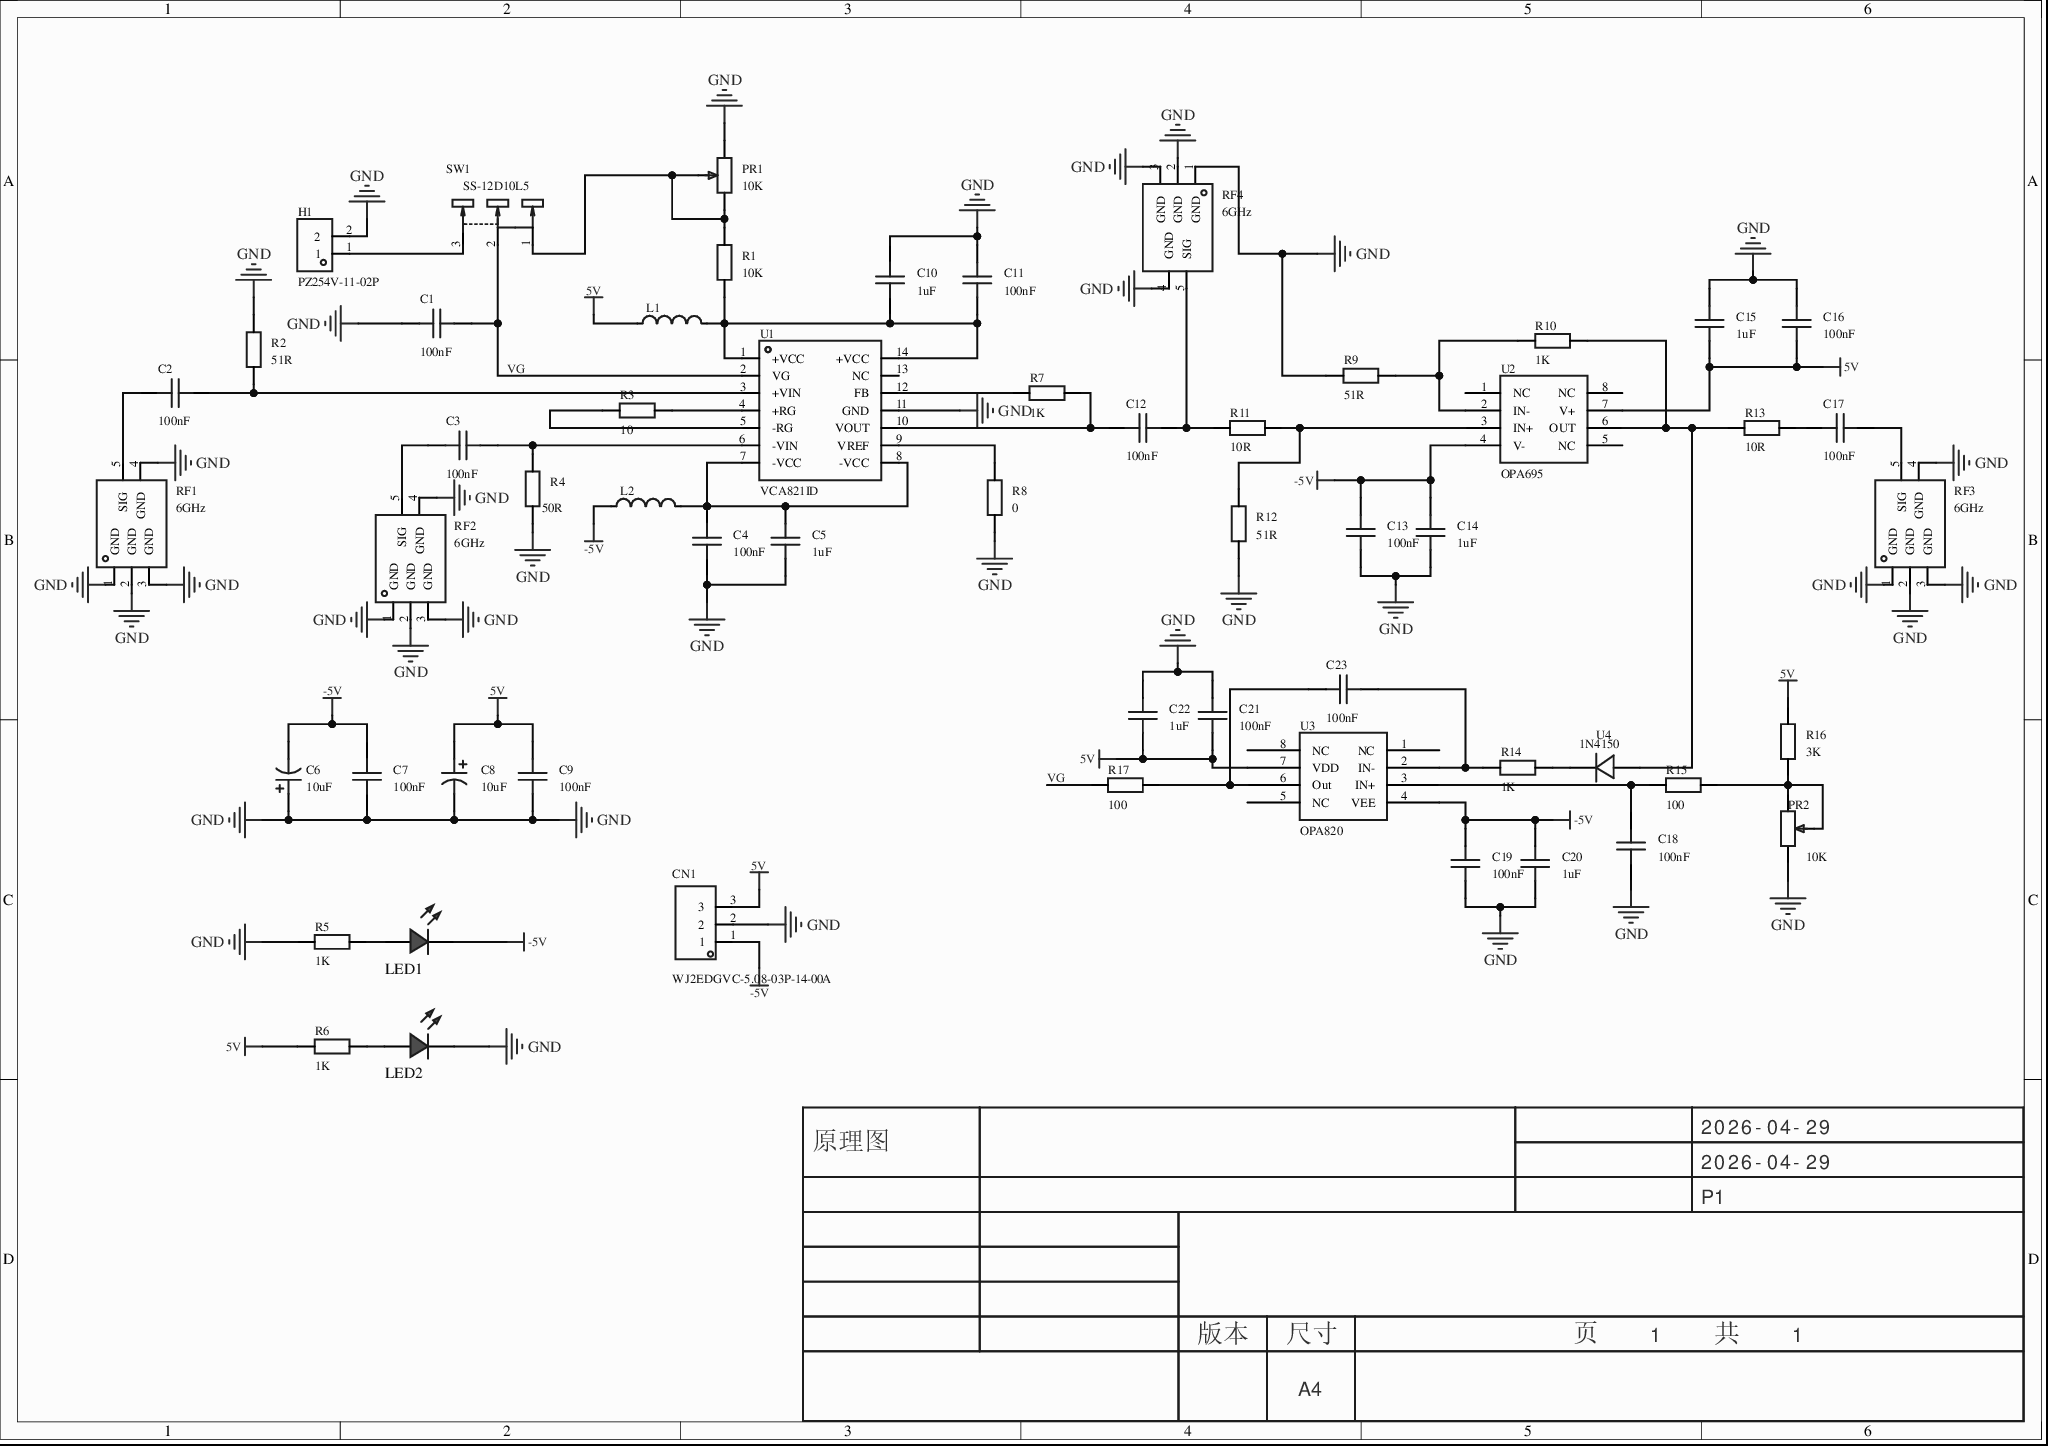
[diagram p0: MISC52012-3.schdoc]
# Altium project MISC52012-2.PrjPcb
1 sheet, 57 parts. Net scope: global (net labels, ports and power ports of the same name join across sheets).
Board file: MISC52012.pcbdoc

## Sheet MISC52012-3.schdoc
size 297 x 209 mm; Version: V1.0; @Project Name: MISC52012; @Page Count: 1; @Update Date: 2026-04-29; @Create Date: 2026-04-29; @Schematic Name: MISC52012; @Page No: 1; @Board Name: MISC52012; @Create Time: 22:58:53; @Update Time: 22:58:53; Size: A4

### Parts
C1  100nF  [C0603]
C2  100nF  [C0603]
C3  100nF  [C0603]
C4  100nF  [C0603]
C5  1uF  [C0603]
C6  10uF  [CAP-TH_BD5.0-P2.00-D0.5-FD-A]
C7  100nF  [C0603]
C8  10uF  [CAP-TH_BD5.0-P2.00-D0.5-FD-A]
C9  100nF  [C0603]
C10  1uF  [C0603]
C11  100nF  [C0603]
C12  100nF  [C0603]
C13  100nF  [C0603]
C14  1uF  [C0603]
C15  1uF  [C0603]
C16  100nF  [C0603]
C17  100nF  [C0603]
C18  100nF  [C0603]
C19  100nF  [C0603]
C20  1uF  [C0603]
C21  100nF  [C0603]
C22  1uF  [C0603]
C23  100nF  [C0603]
CN1  WJ2EDGVC-5.08-03P-14-00A  [CONN-TH_3P-P5.08-WJ2EDGVC-3P]
H1  PZ254V-11-02P  [HDR-TH_2P-P2.54-V-M]
L1  10uH  [L0603]  (value not drawn)
L2  10uH  [L0603]  (value not drawn)
LED1  (no value)  [LED_0603]
LED2  (no value)  [LED_0603]
PR1  10K  [R_3386P]
PR2  10K  [R_3386P]
R1  10K  [R0603]
R2  51R  [R0603]
R3  10  [R0603]
R4  50R  [R0603]
R5  1K  [R0603]
R6  1K  [R0603]
R7  1K  [R0603]
R8  0  [R0603]
R9  51R  [R0603]
R10  1K  [R0603]
R11  10R  [R0603]
R12  51R  [R0603]
R13  10R  [R0603]
R14  1K  [R0603]
R15  100  [R0603]
R16  3K  [R0603]
R17  100  [R0603]
RF1  6GHz  [SMA-SMD_BWSMA-KE-P001]
RF2  6GHz  [SMA-SMD_BWSMA-KE-P001]
RF3  6GHz  [SMA-SMD_BWSMA-KE-P001]
RF4  6GHz  [SMA-SMD_BWSMA-KE-P001]
SW1  SS-12D10L5  [SW-TH_SS-12D10L5]
U1  VCA821ID  [SOIC-14_L8.7-W3.9-P1.27-LS6.0-BL]
U2  OPA695  [SOIC-8]
U3  OPA820  [SOP8]
U4  1N4150  [SOD-123_L2.7-W1.6-LS3.7-RD-1]

### Nets
5V: C8.1 C9.2 C15.1 C16.1 C21.1 C22.1 CN1.3 L1.1 R6.1 R16.2 U2.7(V+) U3.7(VDD)
-5V: C6.2 C7.2 C13.2 C14.2 C19.2 C20.2 CN1.1 L2.1 LED1.1(C) U2.4(V-) U3.4(VEE)
GND: C1.1 C4.2 C5.1 C6.1 C7.1 C8.2 C9.1 C10.2 C11.2 C13.1 C14.1 C15.2 C16.2 C18.1 C19.1 C20.1 C21.2 C22.2 CN1.2 H1.2 LED2.1(C) PR1.1 PR2.1 R2.2 R4.1 R5.1 R8.1 R9.1 R12.1 RF1.1(GND) RF1.2(GND) RF1.3(GND) RF1.4(GND) RF2.1(GND) RF2.2(GND) RF2.3(GND) RF2.4(GND) RF3.1(GND) RF3.2(GND) RF3.3(GND) RF3.4(GND) RF4.1(GND) RF4.2(GND) RF4.3(GND) RF4.4(GND) U1.11(GND)
VG: C1.2 R17.1 SW1.2 U1.2(VG)
NetC2_1: C2.1 RF1.5(SIG)
NetC2_2: C2.2 R2.1 U1.3(+VIN)
NetC3_1: C3.1 RF2.5(SIG)
NetC3_2: C3.2 R4.2 U1.6(-VIN)
NetC4_1: C4.1 C5.2 L2.2 U1.7(-VCC) U1.8(-VCC)
NetC10_1: C10.1 C11.1 L1.2 R1.1 U1.1(+VCC) U1.14(+VCC)
NetC12_1: C12.1 R7.2 U1.10(VOUT)
NetC12_2: C12.2 R11.1 RF4.5(SIG)
NetC17_1: C17.1 R13.2
NetC17_2: C17.2 RF3.5(SIG)
NetC18_2: C18.2 R15.1 U3.3(IN+)
NetC23_1: C23.1 R14.1 U3.2(IN-)
NetC23_2: C23.2 R17.2 U3.6(Out)
NetH1_1: H1.1 SW1.3
NetLED1_2: LED1.2(A) R5.2
NetLED2_2: LED2.2(A) R6.2
NetPR1_2: PR1.2 PR1.3 R1.2 SW1.1
NetPR2_2: PR2.2 PR2.3 R15.2 R16.1
NetR3_1: R3.1 U1.5(-RG)
NetR3_2: R3.2 U1.4(+RG)
NetR7_1: R7.1 U1.12(FB)
NetR8_2: R8.2 U1.9(VREF)
NetR9_2: R9.2 R10.1 U2.2(IN-)
NetR10_2: R10.2 R13.1 U2.6(OUT) U4.2(A)
NetR11_2: R11.2 R12.2 U2.3(IN+)
NetR14_2: R14.2 U4.1(K)

Not connected (* = marked no-connect by the designer): U1 13(NC)*; U2 1(NC)* 5(NC)* 8(NC)*; U3 1(NC)* 5(NC)* 8(NC)*

### Notes on the sheet
- 2026-04-29
- 原理图
- P1
- 版本
- 尺寸
- A4
- 页    1    共    1

### Library data of the parts
C1-C5 C7 C9-C16 = CAP_0603: ConvertToPcb: yes; SymbolName: Capacitance; ModelId: ac125912035d415993ca9572d50418b1; ModelName: C0603_L1.6-W0.8-H0.8; ModelTransform: 62.992,31.496,0,0,0,0,0,0,0; Device: CAP_0603; AddInBom: yes; Supplier Footprint: 0603; FootprintName: C0603
  C1-C4 C7 C9 C11-C13 C16: Value: 100nF
  C5 C10 C14 C15: Value: 1uF
C6 C8 = ERG50V10M5X11: 容值:10uF;精度:±20%;额定电压:50V;纹波电流:180mA@100kHz;等效串联电阻(ESR):1.3Ω@100kHz;; Manufacturer: JIERR(捷而瑞); AddInBom: yes; ModelId: 230b3bd6484f4b52b9cf74c8bd6c6199; ModelTransform: 197.2437,197.23953,0,0,0,0,0,0,-196.85; Tolerance: ±20%; Voltage Rating: 50V; Pin Spacing: 2mm; Lifetime: 2000hrs@105℃; Symbol: ERG50V10M5X11; Device: ERG50V10M5X11; LCSC Part Name: 10uF ±20% 50V; SupplierPart: C47344184; ManufacturerPart: ERG50V10M5X11; Supplier Footprint: 插件,D5xL11mm; Datasheet: https://item.szlcsc.com/datasheet/ERG50V10M5X11/49556625.html; Supplier: LCSC; ConvertToPcb: yes; FootprintName: CAP-TH_BD5.0-P2.00-D0.5-FD-A; ModelName: CAP-TH_BD5.0-P2.00-D0.5-FD-A; Value: 10uF; Ripple Current: 180mA@100kHz; Equivalent Series Resistance(ESR): 1.3Ω@100kHz; Diameter: 5mm; Height - Seated (Max): 11mm; Operating Temperature: -40℃~+105℃
C17-C23 = CL10B104KB8NNNC: 容值:100nF;精度:±10%;额定电压:50V;温度系数:X7R;; Manufacturer: SAMSUNG(三星); AddInBom: yes; ModelId: ac125912035d415993ca9572d50418b1; ModelName: C0603_L1.6-W0.8-H0.8; ModelTransform: 62.992,31.496,0,0,0,0,0,0,0; Tolerance: ±10%; Voltage Rating: 50V; Temperature Coefficient: X7R; Symbol: CL10B104KB8NNNC; Device: CL10B104KB8NNNC; LCSC Part Name: 100nF ±10% 50V; ManufacturerPart: CL10B104KB8NNNC; Supplier Footprint: 0603; JLCPCB Part Class: Extended Part; Datasheet: https://item.szlcsc.com/datasheet/CL10B104KB8NNNC/1943.html; Supplier: LCSC; ConvertToPcb: yes; FootprintName: C0603
  C17-C19 C21 C23: SupplierPart: C1591; Value: 100nF
  C20 C22: Value: 1uF
CN1 = WJ2EDGVC-5.08-03P-14-00A: 连接器类型:板端/插座-闭口;固定方式:卡扣固定;结构:1x3P;间距:5.08mm;颜色:绿色;安装方式:直插;排数:1;每排PIN数:3;额定电流:10A;额定电压:300V;线规 - AWG:-;线规 - 平方毫米:-;工作温度:-40℃~+105℃;; Manufacturer: KANGNEX(康奈克斯电气); Symbol: WJ2EDGVC-3P; AddInBom: yes; ModelId: e882f8e8ed7147e981563fc403497786; ModelTransform: 674.8018,326.771,0,0,0,0,0,17.323,-157.48; Number of Positions or Pins: 1x3P; Pitch: 5.08mm; Number of PINs Per Row: 3; Current Rating: 10A; Voltage Rating (Max): 300V; Device: WJ2EDGVC-5.08-03P-14-00A; LCSC Part Name: 卡扣固定 1x3P 5.08mm 排数:1 每排P数:3; SupplierPart: C8412; ManufacturerPart: WJ2EDGVC-5.08-03P-14-00A; Supplier Footprint: 插件,P=5.08mm; JLCPCB Part Class: 扩展库; Datasheet: https://item.szlcsc.com/datasheet/WJ2EDGVC-5.08-03P-14-00A/8906.html; Supplier: LCSC; ConvertToPcb: yes; FootprintName: CONN-TH_3P-P5.08-WJ2EDGVC-3P; ModelName: CONN-TH_3P-P5.08-WJ2EDGVC-3P; Connector Type: 板端/插座-闭口; Termination Style: 卡扣固定; Color: 绿色; Mounting Type: 直插; Number of Pins: 3P; Number of Rows: 1; Wire Gauge - AWG: -; Wire Gauge - mm2: -; Operating Temperature: -40℃~+105℃; Connection Type: -; Outlet Direction (Vertical Basis): -
H1 = PZ254V-11-02P: 插针结构:1x2P;间距:2.54mm;行距:-;圆针/方针:方针;安装方式:直插;排数:单排;总PIN位数:2P;额定电流:3A;额定电压:250V;配合针长度:6mm;塑高:2.5mm;端接针长度:3mm;触头材质:黄铜;触头镀层:-;工作温度:-40℃~+105℃;颜色:黑色;; Manufacturer: XFCN(兴飞); AddInBom: yes; ModelId: e35305ec3aa84b66b849f914b715e73f; ModelName: HDR2.54-M-LI-1X2P; ModelTransform: 200,100,0,0,0,0,0,0,-118.11; Pin Structure: 1x2P; Pitch: 2.54mm; Circluar Pins/Square Pins: 方针; Current Rating: 3A; Voltage Rating (Max): 250V; Symbol: PZ254V-11-02P; Device: PZ254V-11-02P; LCSC Part Name: 1x2P 间距:2.54mm 方针 直插; SupplierPart: C492401; ManufacturerPart: PZ254V-11-02P; Supplier Footprint: 插件,P=2.54mm; Datasheet: https://item.szlcsc.com/datasheet/PZ254V-11-02P/502957.html; Supplier: LCSC; ConvertToPcb: yes; FootprintName: HDR-TH_2P-P2.54-V-M; Row Spacing: -; Mounting Type: 直插; Number of Rows: 单排; Number of Pins: 2P; Length of Mating Pin: 6mm; Insulation Height: 2.5mm; Length of End Connection Pin: 3mm; Contact Material: 黄铜; Contact Plating: -; Operating Temperature: -40℃~+105℃; Color: 黑色
L1 L2 = L_0603: Symbol: SDFL1608S100KTF; AddInBom: yes; ModelId: 2bc5ec593d464d6ba9807aec0b5673c2; ModelName: L0603_L1.6-W0.8-H0.5_BEAD; ModelTransform: 62.992,31.496,0,180,0,0,0.094,0.629,0; Device: L_0603; Supplier Footprint: L0603; ConvertToPcb: yes; FootprintName: L0603; Value: 10uH
LED1 LED2 = LED_0603-R: Symbol: LED_R; Convert to PCB: yes; 3D Model: dd8257b0d61a4cd7b68939a056e08095; 3D Model Transform: 58.72,29.4,22.03,0,0,0,0,0,0; ModelName: LED-0603_R; Device: LED_0603-R; Add into BOM: yes; Supplier Footprint: 0603; FootprintName: LED_0603
PR1 PR2 = R_3386P: Symbol: 3386P-1-103LF; ConvertToPcb: yes; ModelId: 6a25d8a4450b4318959c1cd98efa6b0c0819f05c4eef4c71ace90d822a990e87; ModelName: RES-ADJ-TH_3P-L9.5-W9.5-P2.54-BR-BS; ModelTransform: 375.19,375.19,387,-90,0,0,0,0,-197; Device: R_3386P; AddInBom: yes; FootprintName: R_3386P; Value: 10K; Supplier Footprint: 直插
R1-R17 = Res_0603: ConvertToPcb: yes; SymbolName: 电阻; ModelId: fc143cca1e79419f9cd78b61e9279f08; ModelTransform: 31.8897,63.7794,0,90,0,0,0,0,0; Device: Res_0603; AddInBom: yes; Supplier Footprint: 0603; FootprintName: R0603; ModelName: R0603
  R1: Value: 10K
  R2 R9 R12: Value: 51R
  R3: Value: 10
  R4: Value: 50R
  R5-R7 R10 R14: Value: 1K
  R8: Value: 0
  R11 R13: Value: 10R
  R15 R17: Value: 100
  R16: Value: 3K
RF1-RF4 = SMA-KHD9A: 连接器类型:板端;接口类型:内孔;端口数量:1;接口长度/高度:8mm;频率:6GHz;射频系列:SMA;阻抗:50Ω;样式:偏脚;; Manufacturer: cntitle(中戈泰斗); AddInBom: yes; ModelId: 45bafb7576014fe1be3aebd244b0ca8e0819f05c4eef4c71ace90d822a990e87; ModelName: SMA-TH_5P-L6.5-W6.5-H9.5_BWSMA-KE-P001; ModelTransform: 255.905,255.905,0,180,0,90,-23.62,0,17.717; Connector Type: 板端; Interface: 内孔; Number of Ports: 1; Interface Length/Height: 8mm; RF Series: SMA; Impedance: 50Ω; Style: 偏脚; Symbol: SMA-KHD9A; Device: SMA-KHD9A; LCSC Part Name: 内孔 SMA 偏脚; SupplierPart: C20415779; ManufacturerPart: SMA-KHD9A; Supplier Footprint: 插件; JLCPCB Part Class: Extended Part; Datasheet: https://item.szlcsc.com/datasheet/SMA-KHD9A/21743961.html; Supplier: LCSC; ConvertToPcb: yes; FootprintName: SMA-SMD_BWSMA-KE-P001; Value: 6GHz
SW1 = SS-12D10L5: 电路结构:单刀双掷;安装方式:直插;开关颜色:黑色;额定电流:3A;额定电压:125V;工作寿命:1万次;; Manufacturer: XKB Connection(中国星坤); AddInBom: yes; ModelId: c49f07a32c154ec8ad7cf47670a53981; ModelName: SW-TH_L13.0-W6.8-H6.4-P4.7; ModelTransform: 511.81394,267.716,0,0,0,0,0,0,-220.472; Circuit: 单刀双掷; Actuator Style: 矩形柱状; Switch Height: 6.4mm; Actuator Color: 黑色; Current Rating: 3A; Voltage Rating: 125V; Life: 1万次; Symbol: SS-12D10L5; Device: SS-12D10L5; LCSC Part Name: 柄长5mm 直插双档 滑动开关; SupplierPart: C319012; ManufacturerPart: SS-12D10L5; Supplier Footprint: 插件,13x6.8mm; JLCPCB Part Class: 扩展库; Datasheet: https://item.szlcsc.com/datasheet/SS-12D10L5/300104.html; Supplier: LCSC; ConvertToPcb: yes; FootprintName: SW-TH_SS-12D10L5; Termination Style: PC引脚; Length: 13mm; Width: 6.8mm; Mounting Type: 直插; Operating Temperature: -40℃~+85℃
U1 = VCA821ID: 放大器类型:VGA;通道数:单路;增益:32dB;带宽(-3db):710MHz;压摆率(SR):2500V/us;轨到轨:-;输出电流:90mA;; Manufacturer: TI(德州仪器); AddInBom: yes; ModelId: 8dbf5b715d42428c85558507ae5a252b; ModelName: SOIC-14_L8.6-W3.9-H1.8-LS6.0-P1.27; ModelTransform: 338.583,236.22,0,0,0,0,0,0.001,0; Amplifier Type: VGA; Number of Channels: 单路; Gain: 32dB; -3dB Bandwidth: 710MHz; Output Current: 90mA; Current - Supply: 34mA; Symbol: VCA821ID; Device: VCA821ID; LCSC Part Name: VCA821ID; SupplierPart: C2866982; ManufacturerPart: VCA821ID; Supplier Footprint: SOIC-14; JLCPCB Part Class: 扩展库; Datasheet: https://www.ti.com/cn/lit/gpn/vca821; Supplier: LCSC; ConvertToPcb: yes; FootprintName: SOIC-14_L8.7-W3.9-P1.27-LS6.0-BL; Slew Rate: 2500V/us; Rail to Rail: -; Operating Temperature: -40℃~+85℃
U2 = OPA695: AddInBom: yes; Origin Footprint 2: DIP8; Device: OPA695; ConvertToPcb: yes; SymbolName: OPA695; FootprintName: SOIC-8
U3 = OPA820: AddInBom: yes; Device: OPA820; ConvertToPcb: yes; SymbolName: OPA820; FootprintName: SOP8
U4 = 1N4150W-E3-18: 二极管配置:1个独立式;正向压降(Vf):1V@200mA;直流反向耐压(Vr):50V;整流电流:200mA;反向恢复时间(Trr):4ns;; Manufacturer: VISHAY(威世); AddInBom: yes; ModelId: 528459655f7d4601a76356f3191c812b; ModelTransform: 151.575,66.929,0,0,0,0,0,0,0; Diode Configuration: 1个独立式; Voltage - DC Reverse(Vr): 50V; Current - Rectified: 200mA; Pd - Power Dissipation: 410mW; Reverse Leakage Current (Ir): 100nA@50V; Reverse Recovery Time (trr): 4ns; Operating Junction Temperature Range: -55℃~+150℃; Symbol: 1N4150W-E3-18; Manufacturer Part: 1N4150; Device: 1N4150W-E3-18; LCSC Part Name: 50V 200mA; SupplierPart: C5345077; Supplier Footprint: SOD-123; JLCPCB Part Class: 扩展库; Datasheet: https://item.szlcsc.com/datasheet/1N4150W-E3-18/6123465.html; Supplier: LCSC; ConvertToPcb: yes; FootprintName: SOD-123_L2.7-W1.6-LS3.7-RD-1; ModelName: SOD-123_L2.7-W1.6-LS3.7-RD-1; Voltage - Forward(Vf@If): 1V@200mA